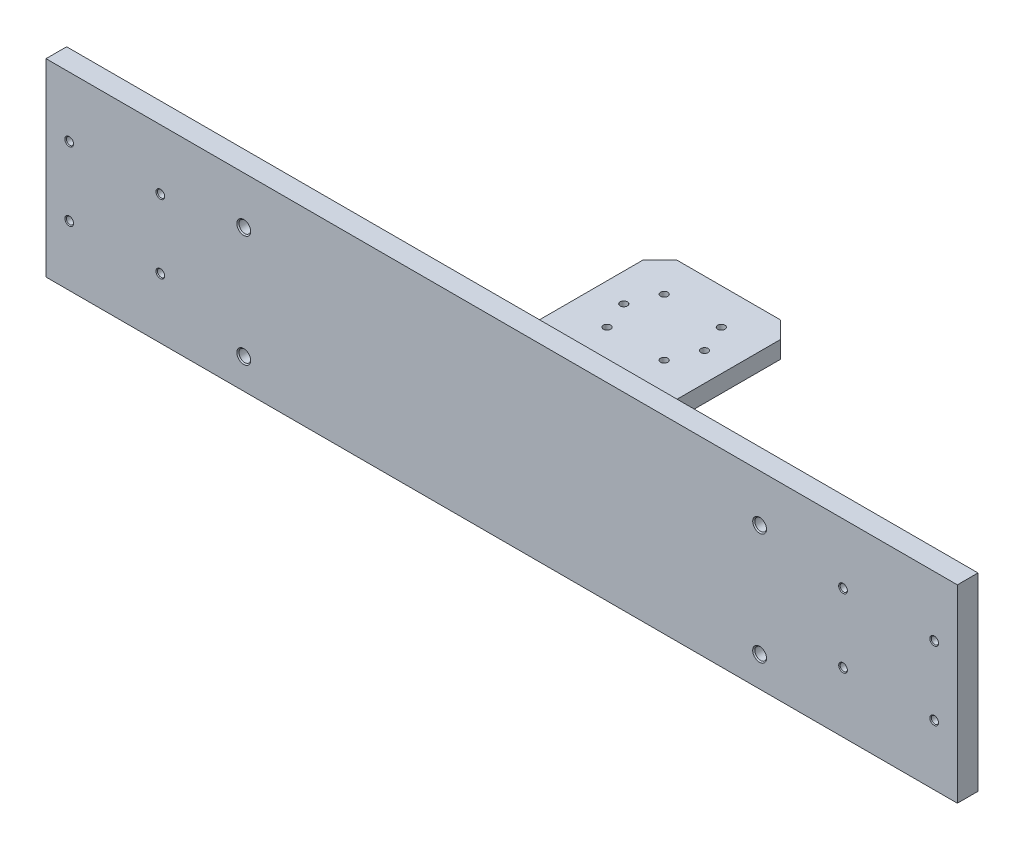
from build123d import *

# Parameters (mm, degrees)
SKETCH1_W                   = 80
SKETCH1_H                   = 120
BOSS_EXTRUDE1_DEPTH         = 10
SKETCH2_W                   = 530
SKETCH2_H                   = 110
BOSS_EXTRUDE2_DEPTH         = 12
CHAMFER1_SIZE               = 10
CUT_EXTRUDE1_DEPTH          = 303.553620593
CUT_EXTRUDE1_DEPTH_BACK     = 303.553620593
SKETCH3_R                   = 2.1
M5_TAPPED_HOLE1_D           = 4.2
M5_TAPPED_HOLE1_DEPTH       = 12.4
M5_TAPPED_HOLE1_CSINK_D     = 5.05
M5_TAPPED_HOLE1_CSINK_ANGLE = 90
M5_TAPPED_HOLE1_TIP         = 1.2618073
M8_TAPPED_HOLE1_D           = 6.8
M8_TAPPED_HOLE1_DEPTH       = 22.25
M8_TAPPED_HOLE1_CSINK_D     = 8.05
M8_TAPPED_HOLE1_CSINK_ANGLE = 90
M8_TAPPED_HOLE1_TIP         = 2.042926105


with BuildPart() as part:
    # Sketch1 → Boss-Extrude1 (new body)
    with BuildSketch(Plane(origin=(0, 0, 0), x_dir=(1, 0, 0), z_dir=(0, 1, 0))):
        with Locations((-10, -38.967082208)):
            Rectangle(SKETCH1_W, SKETCH1_H)
    extrude(amount=BOSS_EXTRUDE1_DEPTH)

    # Sketch2 → Boss-Extrude2 (add)
    with BuildSketch(Plane.XY.offset(98.967082208)):
        with Locations((-10, 5)):
            Rectangle(SKETCH2_W, SKETCH2_H)
    extrude(amount=BOSS_EXTRUDE2_DEPTH)

    # Chamfer1
    chamfer1_edges = [part.edges().sort_by_distance(p)[0] for p in [
        (-50, 5, -21.032917792),
        (30, 5, -21.032917792),
    ]]
    chamfer(chamfer1_edges, length=CHAMFER1_SIZE)

    # Sketch3 → Cut-Extrude1 (cut, two sides: drawn at the far end of the back side and taken through both)
    with BuildSketch(Plane(origin=(0, 10, 0), x_dir=(1, 0, 0), z_dir=(0, 1, 0)).offset(-CUT_EXTRUDE1_DEPTH_BACK)):
        with Locations(Location((6.617009358, 0.14992715, 0), (0, 0, 270))):
            Circle(SKETCH3_R)
        with Locations(Location((13.499999853, -16.467082208, 0), (0, 0, 270))):
            Circle(SKETCH3_R)
        with Locations(Location((6.617009358, -33.084091566, 0), (0, 0, 270))):
            Circle(SKETCH3_R)
        with Locations(Location((-26.617009358, -33.084091566, 0), (0, 0, 270))):
            Circle(SKETCH3_R)
        with Locations(Location((-33.499999853, -16.467082208, 0), (0, 0, 270))):
            Circle(SKETCH3_R)
        with Locations(Location((-26.617009358, 0.14992715, 0), (0, 0, 270))):
            Circle(SKETCH3_R)
    extrude(amount=CUT_EXTRUDE1_DEPTH + CUT_EXTRUDE1_DEPTH_BACK, mode=Mode.SUBTRACT)

    # M5 Tapped Hole1
    with Locations(Plane.XY.offset(110.967082208)):
        with Locations((-261.5, 25), (-261.5, -15), (-208.5, 25), (-208.5, -15), (188.5, -15), (188.5, 25), (241.5, -15), (241.5, 25)):
            CounterSinkHole(M5_TAPPED_HOLE1_D / 2, M5_TAPPED_HOLE1_CSINK_D / 2, depth=M5_TAPPED_HOLE1_DEPTH, counter_sink_angle=M5_TAPPED_HOLE1_CSINK_ANGLE)
            with Locations((0, 0, -(M5_TAPPED_HOLE1_DEPTH + M5_TAPPED_HOLE1_TIP / 2))):  # 118° drill point
                Cone(0, M5_TAPPED_HOLE1_D / 2, M5_TAPPED_HOLE1_TIP, mode=Mode.SUBTRACT)

    # M8 Tapped Hole1
    with Locations(Plane.XY.offset(110.967082208)):
        with Locations((-160, 32.5), (-160, -32.5), (140, 32.5), (140, -32.5)):
            CounterSinkHole(M8_TAPPED_HOLE1_D / 2, M8_TAPPED_HOLE1_CSINK_D / 2, depth=M8_TAPPED_HOLE1_DEPTH, counter_sink_angle=M8_TAPPED_HOLE1_CSINK_ANGLE)
            with Locations((0, 0, -(M8_TAPPED_HOLE1_DEPTH + M8_TAPPED_HOLE1_TIP / 2))):  # 118° drill point
                Cone(0, M8_TAPPED_HOLE1_D / 2, M8_TAPPED_HOLE1_TIP, mode=Mode.SUBTRACT)


solid = part.part
